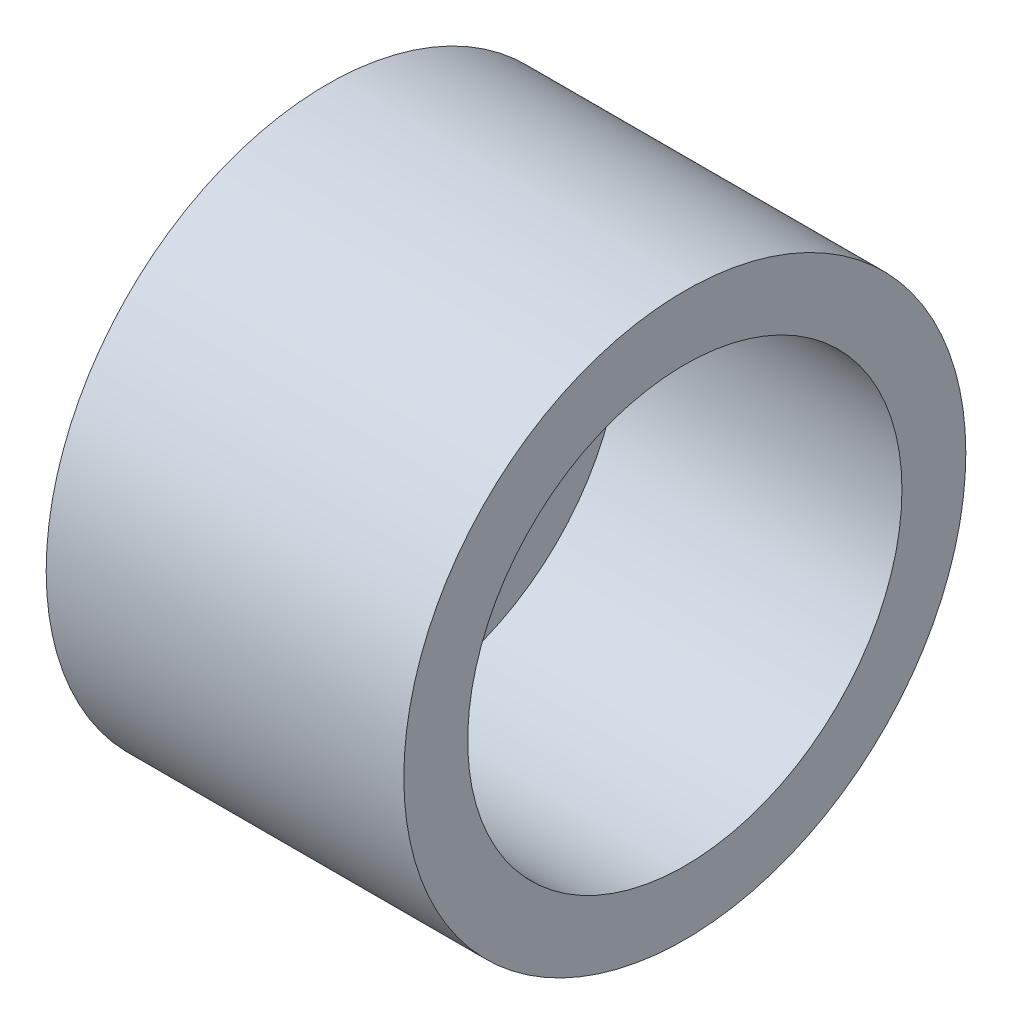
SolidWorks part; units mm, degrees
ref_plane "Front Plane" through (0, 0, 0) normal (0, 0, 1) x (1, 0, 0)
ref_plane "Top Plane" through (0, 0, 0) normal (0, 1, 0) x (1, 0, 0)
ref_plane "Right Plane" through (0, 0, 0) normal (1, 0, 0) x (0, 0, -1)
other "Configuration Table"
sketch "Sketch1" plane through (0, 0, 0) normal (1, 0, 0) x (0, 0, -1)
  circle A0 centre (0, 0) radius 5.5
  circle A1 centre (0, 0) radius 2.75
  dimension "D1" = 11
  dimension "D2" = 5.5
extrude "Boss-Extrude1" add sketch "Sketch1" along normal blind 7
sketch "Sketch2" plane through (7, 0, 0) normal (1, 0, 0) x (0, 0, -1)
  circle A0 centre (0, 0) radius 4.25
  dimension "D1" = 8.5
extrude "Cut-Extrude1" cut sketch "Sketch2" against normal blind 5.5
